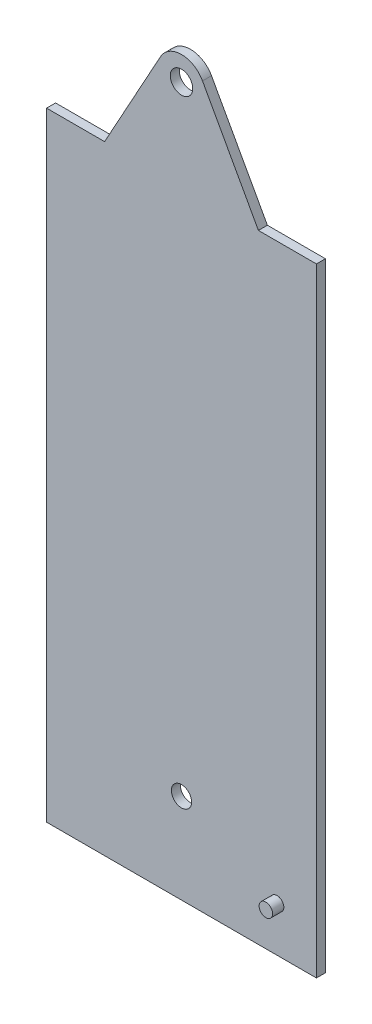
from build123d import *

# Parameters (mm, degrees)
SKETCH1_R           = 10
SKETCH1_R_2         = 9
BOSS_EXTRUDE1_DEPTH = 8
SKETCH2_R           = 6
BOSS_EXTRUDE2_DEPTH = 10


with BuildPart() as part:
    # Sketch1 → Boss-Extrude1 (new body)
    with BuildSketch(Plane.XY):
        with BuildLine():
            Line((-120, 550), (-68.4, 550))
            Line((-68.4, 550), (-18.684224353, 640.288176603))
            ThreePointArc((-18.684224353, 640.288176603), (0, 651.329482354), (18.684224353, 640.288176603))
            Line((18.684224353, 640.288176603), (68.4, 550))
            Line((68.4, 550), (120, 550))
            Line((120, 550), (120, 0))
            Line((120, 0), (-120, 0))
            Line((-120, 0), (-120, 550))
        make_face()
        with Locations((0, 630)):
            Circle(SKETCH1_R, mode=Mode.SUBTRACT)
        with Locations((0, 80)):
            Circle(SKETCH1_R_2, mode=Mode.SUBTRACT)
    extrude(amount=BOSS_EXTRUDE1_DEPTH)

    # Sketch2 → Boss-Extrude2 (add)
    with BuildSketch(Plane.XY.offset(8)):
        with Locations((85, 40)):
            Circle(SKETCH2_R)
    extrude(amount=BOSS_EXTRUDE2_DEPTH)


solid = part.part
